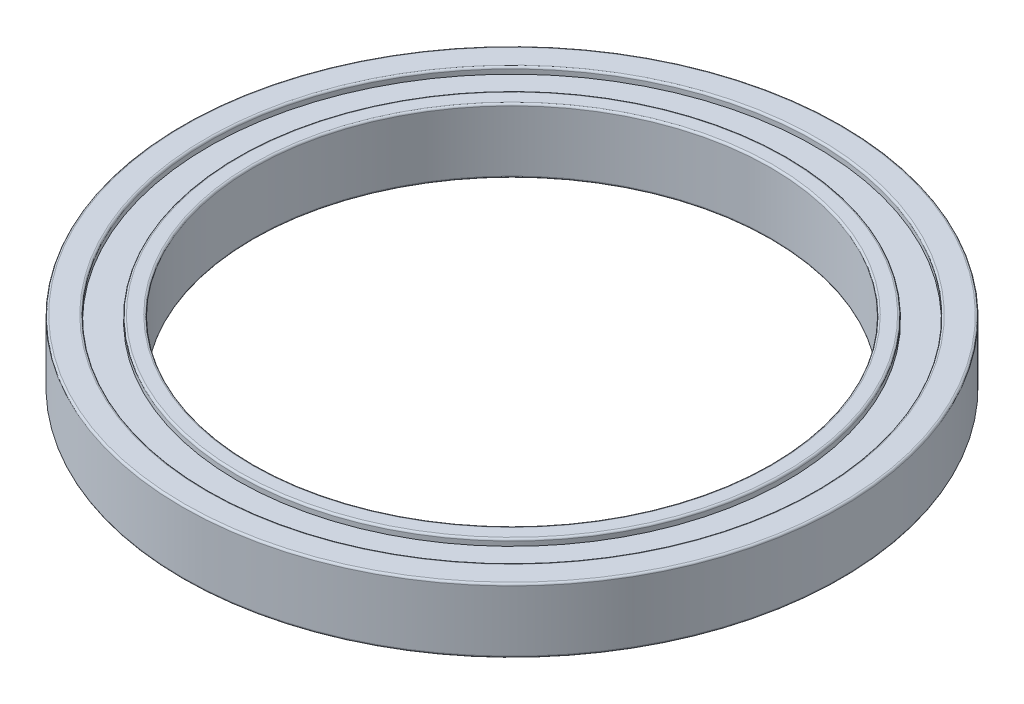
SolidWorks part; units mm, degrees
material "镀铬不锈钢"
ref_plane "前视基准面" through (0, 0, 0) normal (0, 0, 1) x (1, 0, 0)
ref_plane "上视基准面" through (0, 0, 0) normal (0, 1, 0) x (1, 0, 0)
ref_plane "右视基准面" through (0, 0, 0) normal (1, 0, 0) x (0, 0, -1)
sketch "草图1" plane through (0, 0, 0) normal (0, 1, 0) x (1, 0, 0)
  circle A0 centre (0, 0) radius 25.5
  circle A1 centre (0, 0) radius 20
  dimension "D1" = 51
  dimension "D2" = 40
extrude "凸台-拉伸1" add sketch "草图1" along normal mid plane 5
ref_axis "中心轴" through (0, 2.5, 0) along (0, -1, 0)
sketch "草图2" plane through (0, 2.5, 0) normal (0, 1, 0) x (1, 0, 0)
  circle A0 centre (0, 0) radius 23.5
  circle A1 centre (0, 0) radius 21.25
  dimension "D1" = 42.5
  dimension "D2" = 47
extrude "轴肩-上" cut sketch "草图2" against normal blind 0.5
sketch "草图3" plane through (0, -2.5, 0) normal (0, -1, 0) x (1, 0, 0)
  circle A1 centre (0, 0) radius 21.25
  circle A2 centre (0, 0) radius 21.25
  circle A3 centre (0, 0) radius 23.5
  circle A4 centre (0, 0) radius 23.5
  dimension "D1" = 0
  dimension "D2" = 0
extrude "轴肩-下" cut sketch "草图3" against normal blind 0.5
sketch "草图4" plane through (0, 0, 0) normal (0, 0, 1) x (1, 0, 0)
  line L0 (-22.35, 0) -> (0, 0) construction
  circle A0 centre (-22.35, 0) radius 0.75
  point P4 (0, 0)
  dimension "D2" = 1.5
  dimension "D1" = 22.35
revolve "滚道" cut sketch "草图4" angle 360 about axis through (0, 2.5, 0) along (0, -1, 0)
sketch "草图5" plane through (0, 0, 0) normal (0, 0, 1) x (1, 0, 0)
  circle A0 centre (0, 0) radius 0.5
  dimension "D1" = 1
extrude "切除-拉伸1" cut sketch "草图5" against normal through all from offset 22.35 offset against normal yes
fillet "R0.15 圆角" radius 0.15 8 edges at (0, -2.5, -21.25) (0, -2.5, 20) (0, -2.5, 25.5) (0, -2.5, -23.5) (0, 2.5, 21.25) (0, 2.5, 20) (0, 2.5, 25.5) (0, 2.5, 23.5)
